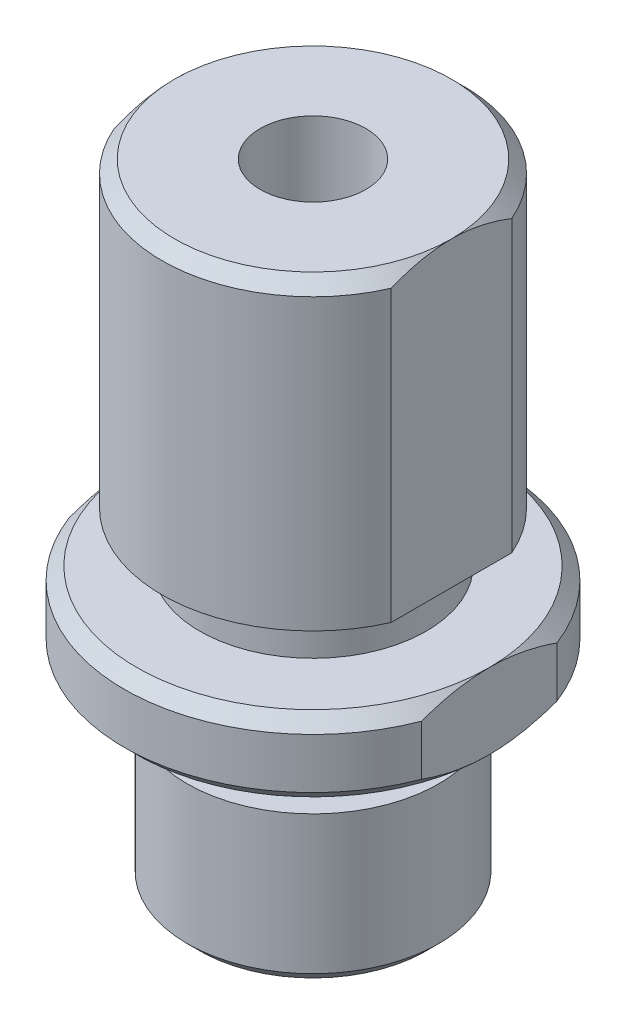
SolidWorks part; units mm, degrees
ref_plane "前视基准面" through (0, 0, 0) normal (0, 0, 1) x (1, 0, 0)
ref_plane "上视基准面" through (0, 0, 0) normal (0, 1, 0) x (1, 0, 0)
ref_plane "右视基准面" through (0, 0, 0) normal (1, 0, 0) x (0, 0, -1)
sketch "草图1" plane through (0, 0, 0) normal (0, 1, 0) x (1, 0, 0)
  circle A0 centre (0, 0) radius 6
  dimension "D1" = 12
extrude "凸台-拉伸1" add sketch "草图1" against normal blind 14
sketch "草图2" plane through (0, -14, 0) normal (0, -1, 0) x (1, 0, 0)
  circle A0 centre (0, 0) radius 7.5
  dimension "D1" = 15
extrude "凸台-拉伸2" add sketch "草图2" along normal blind 3
sketch "草图3" plane through (0, -17, 0) normal (0, -1, 0) x (1, 0, 0)
  circle A0 centre (0, 0) radius 5
  dimension "D1" = 10
extrude "凸台-拉伸3" add sketch "草图3" along normal blind 8
cosmetic thread "装饰螺纹线1" parameters "D2"=9
sketch "草图4" plane through (0, -25, 0) normal (0, -1, 0) x (1, 0, 0)
  circle A0 centre (0, 0) radius 3.5
  dimension "D1" = 7
extrude "凸台-拉伸4" [suppressed] add sketch "草图4" along normal blind 5
sketch "草图8" plane through (0, 0, 0) normal (0, -1, 0) x (1, 0, 0)
  circle A0 centre (0, 0) radius 2.1
  dimension "D1" = 4.2
extrude "切除-拉伸1" cut sketch "草图8" along normal through all
cosmetic thread "装饰螺纹线2" parameters "D1"=12, "D2"=5
chamfer "倒角1" distance 0.5 angle 45 3 edges at (0, -17, -7.5) (0, -14, -7.5) (0, 0, 6)
sketch "草图9" plane through (0, 0, 0) normal (0, 0, 1) x (1, 0, 0)
  line L1 (21.7723, -4.1347) -> (7, -4.1347)
  line L2 (21.7723, -4.1347) -> (21.7723, -17.6867)
  line L3 (21.7723, -17.6867) -> (7, -17.6867)
  line L4 (7, -4.1347) -> (7, -17.6867)
  line L5 (21.7723, -4.1347) -> (7, -17.6867) construction
  line L6 (21.7723, -17.6867) -> (7, -4.1347) construction
  point P0 (14.3862, -10.9107)
  dimension "D1" = 0.5
extrude "切除-拉伸2" cut sketch "草图9" against normal mid plane 9
mirror "镜向1" about plane through (0, 0, 0) normal (1, 0, 0) of "切除-拉伸2"
chamfer "倒角2" distance 0.5 angle 45 1 edges at (0, -25, -5)
sketch "草图11" plane through (0, 0, 0) normal (0, 0, 1) x (1, 0, 0)
  line L0 (7, -14) -> (-7, -14) construction
  line L1 (15.1439, 13.5415) -> (5.5, 13.5415)
  line L2 (15.1439, 13.5415) -> (15.1439, -14)
  line L3 (15.1439, -14) -> (5.5, -14)
  line L4 (5.5, 13.5415) -> (5.5, -14)
  line L5 (15.1439, 13.5415) -> (5.5, -14) construction
  line L6 (15.1439, -14) -> (5.5, 13.5415) construction
  line L7 (-19.357, 13.5415) -> (-5.5, 13.5415)
  line L8 (-19.357, 13.5415) -> (-19.357, -14)
  line L9 (-19.357, -14) -> (-5.5, -14)
  line L10 (-5.5, 13.5415) -> (-5.5, -14)
  line L11 (-19.357, 13.5415) -> (-5.5, -14) construction
  line L12 (-19.357, -14) -> (-5.5, 13.5415) construction
  line L13 (-6, -0.5) -> (-6, -14) construction
  line L14 (6, -14) -> (6, -0.5) construction
  point P0 (10.3219, -0.2292)
  point P5 (-12.4285, -0.2292)
  dimension "D1" = 0.5
  dimension "D2" = 0.5
extrude "切除-拉伸3" cut sketch "草图11" against normal mid plane 20
sketch "草图12" plane through (0, 0, 0) normal (0, 0, 1) x (1, 0, 0)
  line L0 (-7, -17) -> (7, -17) construction
  line L1 (-13.2928, -17) -> (-4, -17)
  line L2 (-13.2928, -17) -> (-13.2928, -19)
  line L3 (-13.2928, -19) -> (-4, -19)
  line L4 (-4, -17) -> (-4, -19)
  line L5 (-13.2928, -17) -> (-4, -19) construction
  line L6 (-13.2928, -19) -> (-4, -17) construction
  line L7 (-5, -17) -> (-5, -24.5) construction
  point P0 (-8.6464, -18)
  dimension "D1" = 1
  dimension "D2" = 2
revolve "切除-旋转2" cut sketch "草图12" angle 360 about axis through (0, -17, 0) along (0, 1, 0)
sketch "草图13" plane through (0, 0, 0) normal (0, 0, 1) x (1, 0, 0)
  line L0 (5.5, -14) -> (-5.5, -14) construction
  line L1 (-11.311, -12) -> (-4.5, -12)
  line L2 (-11.311, -12) -> (-11.311, -14)
  line L3 (-11.311, -14) -> (-4.5, -14)
  line L4 (-4.5, -12) -> (-4.5, -14)
  line L5 (-11.311, -12) -> (-4.5, -14) construction
  line L6 (-11.311, -14) -> (-4.5, -12) construction
  line L7 (-5.5, -14) -> (-5.5, -0.5) construction
  point P0 (-7.9055, -13)
  dimension "D1" = 2
  dimension "D2" = 1
revolve "切除-旋转3" cut sketch "草图13" angle 360 about axis through (0, -14, 0) along (0, 1, 0)
